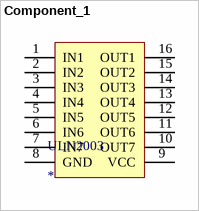
[diagram p0: symbol Component_1]
# Altium schematic symbol library MISC86340-15.SchLib: 1 symbol
Pins are listed as number, name and electrical type; pins without a type are passive.


## Component_1
designator ULN2003
footprint ULN2003
pins: 1 IN1, 2 IN2, 3 IN3, 4 IN4, 5 IN5, 6 IN6, 7 IN7, 8 GND, 9 VCC, 10 OUT7, 11 OUT6, 12 OUT5, 13 OUT4, 14 OUT3, 15 OUT2, 16 OUT1